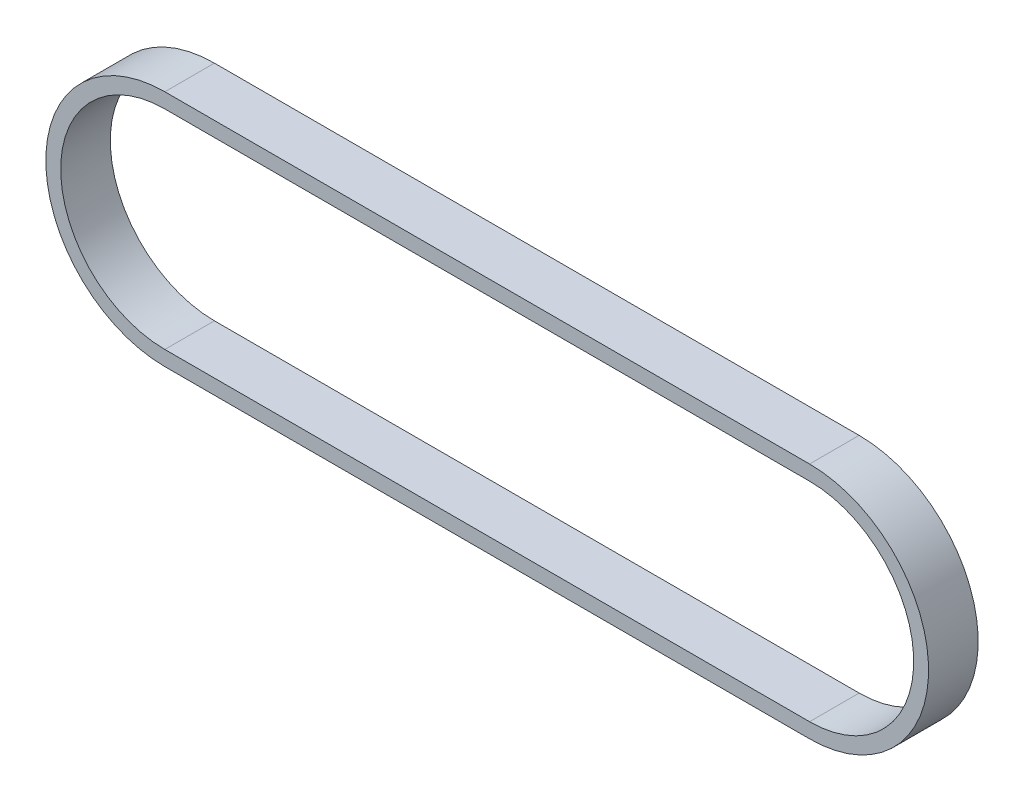
from build123d import *

# Parameters (mm, degrees)
BOSS_EXTRUDE1_DEPTH = 10
SHELL1_T            = -3


with BuildPart() as part:
    # Sketch2 → Boss-Extrude1 (new body)
    with BuildSketch(Plane.XY):
        with BuildLine():
            Line((0, 24), (-130, 24))
            ThreePointArc((-130, 24), (-154, 0), (-130, -24))
            Line((-130, -24), (0, -24))
            ThreePointArc((0, -24), (24, 0), (0, 24))
        make_face()
    extrude(amount=BOSS_EXTRUDE1_DEPTH)

    # Shell1
    shell1_openings = [part.faces().sort_by_distance(p)[0] for p in [
        (-65, 0, 10),
        (-65, 0, 0),
    ]]
    offset(amount=SHELL1_T, openings=shell1_openings, kind=Kind.INTERSECTION)


solid = part.part
